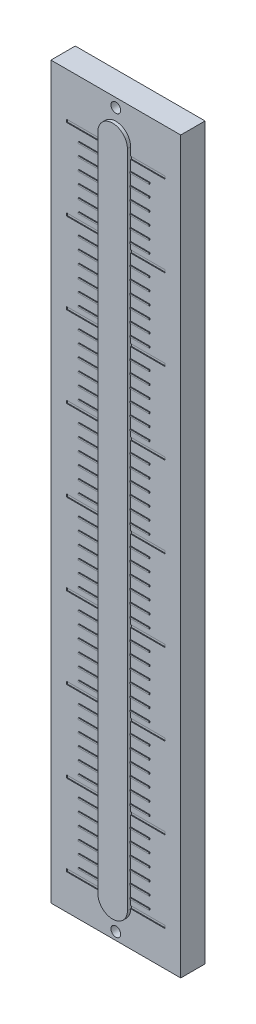
from build123d import *

# Parameters (mm, degrees)
SKETCH1_W           = 80
SKETCH1_H           = 450
SKETCH1_R           = 3
BOSS_EXTRUDE1_DEPTH = 15
BOSS_EXTRUDE2_DEPTH = 2
SKETCH4_W           = 21.329095426
SKETCH4_H           = 1.745927108
SKETCH4_W_2         = 21.306079069
CUT_EXTRUDE1_DEPTH  = 0.5
SKETCH5_W           = 43.65505417
SKETCH5_H           = 0.901431797
BOSS_EXTRUDE3_DEPTH = 0.5
LPATTERN1_COUNT     = 8
LPATTERN1_PITCH     = 50


with BuildPart() as part:
    # Sketch1 → Boss-Extrude1 (new body)
    with BuildSketch(Plane.XY):
        with Locations((40, 225)):
            Rectangle(SKETCH1_W, SKETCH1_H)
        with Locations((40, 444.613221199)):
            Circle(SKETCH1_R, mode=Mode.SUBTRACT)
        with Locations((40, 4.801908956)):
            Circle(SKETCH1_R, mode=Mode.SUBTRACT)
    extrude(amount=BOSS_EXTRUDE1_DEPTH)

    # Sketch2 → Boss-Extrude2 (add)
    with BuildSketch(Plane.XY.offset(15)):
        with BuildLine():
            Line((49.125188537, 428.242835596), (49.125188537, 21.520106217))
            ThreePointArc((49.125188537, 21.520106217), (40.026510765, 12.421428445), (30.927832993, 21.520106217))
            Line((30.927832993, 21.520106217), (30.927832993, 428.242835596))
            ThreePointArc((30.927832993, 428.242835596), (40.026510765, 437.341513368), (49.125188537, 428.242835596))
        make_face()
    extrude(amount=BOSS_EXTRUDE2_DEPTH)

    # Sketch4 → Cut-Extrude1 (cut)
    with BuildSketch(Plane.XY.offset(15)):
        with Locations((59.78973625, 72.393069771)):
            Rectangle(SKETCH4_W, SKETCH4_H)
        with Locations((59.78973625, 22.393069771)):
            Rectangle(SKETCH4_W, SKETCH4_H)
        with Locations((59.78973625, 122.393069771)):
            Rectangle(SKETCH4_W, SKETCH4_H)
        with Locations((59.78973625, 172.393069771)):
            Rectangle(SKETCH4_W, SKETCH4_H)
        with Locations((59.78973625, 222.393069771)):
            Rectangle(SKETCH4_W, SKETCH4_H)
        with Locations((59.78973625, 272.393069771)):
            Rectangle(SKETCH4_W, SKETCH4_H)
        with Locations((59.78973625, 322.393069771)):
            Rectangle(SKETCH4_W, SKETCH4_H)
        with Locations((59.78973625, 372.393069771)):
            Rectangle(SKETCH4_W, SKETCH4_H)
        with Locations((59.78973625, 422.393069771)):
            Rectangle(SKETCH4_W, SKETCH4_H)
        with Locations((20.274793458, 72.393069771)):
            Rectangle(SKETCH4_W_2, SKETCH4_H)
        with Locations((20.274793458, 22.393069771)):
            Rectangle(SKETCH4_W_2, SKETCH4_H)
        with Locations((20.274793458, 122.393069771)):
            Rectangle(SKETCH4_W_2, SKETCH4_H)
        with Locations((20.274793458, 172.393069771)):
            Rectangle(SKETCH4_W_2, SKETCH4_H)
        with Locations((20.274793458, 222.393069771)):
            Rectangle(SKETCH4_W_2, SKETCH4_H)
        with Locations((20.274793458, 272.393069771)):
            Rectangle(SKETCH4_W_2, SKETCH4_H)
        with Locations((20.274793458, 322.393069771)):
            Rectangle(SKETCH4_W_2, SKETCH4_H)
        with Locations((20.274793458, 372.393069771)):
            Rectangle(SKETCH4_W_2, SKETCH4_H)
        with Locations((20.274793458, 422.393069771)):
            Rectangle(SKETCH4_W_2, SKETCH4_H)
    extrude(amount=-CUT_EXTRUDE1_DEPTH, mode=Mode.SUBTRACT)

    # Sketch5 → Boss-Extrude3 (add)
    with BuildSketch(Plane.XY.offset(15)):
        with Locations((39.153473513, 34.819615773)):
            Rectangle(SKETCH5_W, SKETCH5_H)
        with Locations((39.153473513, 27.319615773)):
            Rectangle(SKETCH5_W, SKETCH5_H)
        with Locations((39.153473513, 42.319615773)):
            Rectangle(SKETCH5_W, SKETCH5_H)
        with Locations((39.153473513, 49.819615773)):
            Rectangle(SKETCH5_W, SKETCH5_H)
        with Locations((39.153473513, 57.319615773)):
            Rectangle(SKETCH5_W, SKETCH5_H)
        with Locations((39.153473513, 64.819615773)):
            Rectangle(SKETCH5_W, SKETCH5_H)
    boss_extrude3 = extrude(amount=BOSS_EXTRUDE3_DEPTH)

    # LPattern1: Boss-Extrude3 ×8
    with Locations(*[(0, i * LPATTERN1_PITCH, 0) for i in range(1, LPATTERN1_COUNT)]):
        add(boss_extrude3)


solid = part.part
